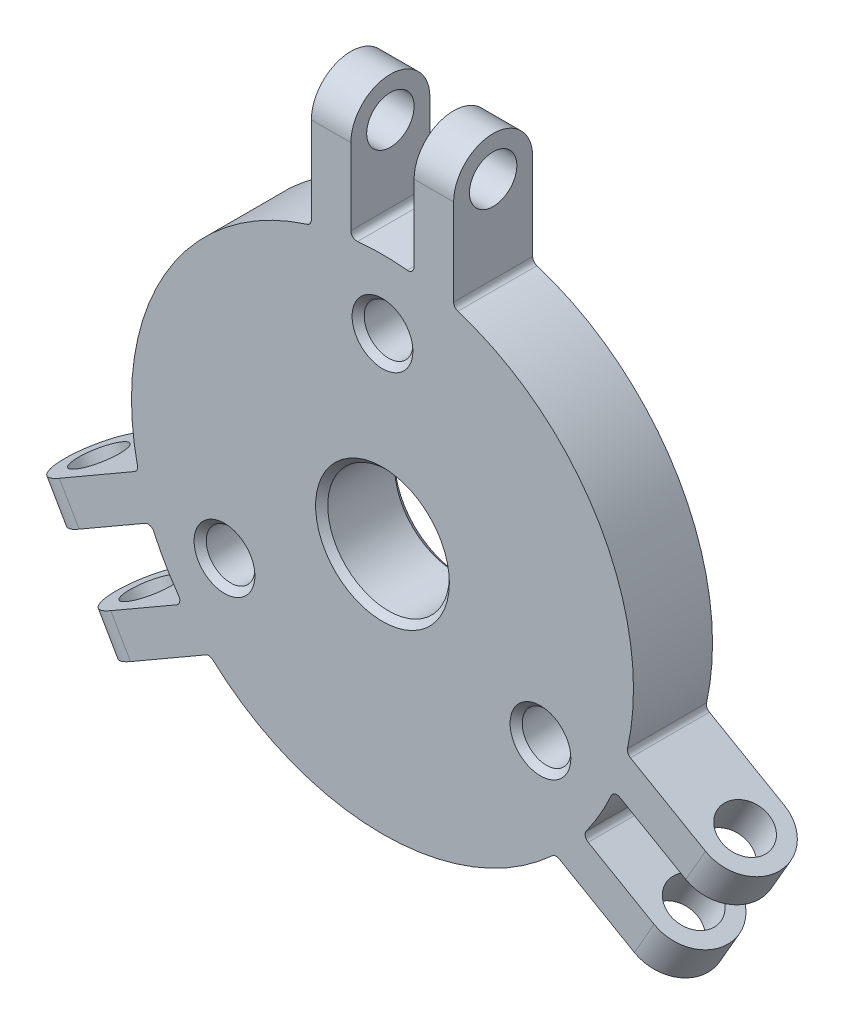
from build123d import *

# Parameters (mm, degrees)
BOSS_EXTRUDE1_DEPTH = 5
SKETCH2_R           = 1.5
CUT_EXTRUDE1_DEPTH  = 15.5
CUT_EXTRUDE3_DEPTH  = 27
CIRPATTERN1_COUNT   = 3
CIRPATTERN2_COUNT   = 3
SCALE_RATIO_1_SCALE = 1.3
SKETCH5_R           = 5
CUT_EXTRUDE4_DEPTH  = 10
CHAMFER1_SIZE       = 0.5
SKETCH8_R           = 2
CUT_EXTRUDE5_DEPTH  = 10
CHAMFER2_SIZE       = 0.5
FILLET1_R           = 0.5


with BuildPart() as part:
    # Sketch1 → Boss-Extrude1 (new body)
    with BuildSketch(Plane.XY):
        with BuildLine():
            Line((-26.5, -17.60918321), (-12.640472866, -9.607381488))
            ThreePointArc((-12.640472866, -9.607381488), (-13.75, -7.938566201), (-14.640472866, -6.143279873))
            Line((-14.640472866, -6.143279873), (-28.5, -14.145081595))
            Line((-28.5, -14.145081595), (-29.75, -11.980018086))
            Line((-29.75, -11.980018086), (-15.436166994, -3.715922747))
            ThreePointArc((-15.436166994, -3.715922747), (-13.75, 7.938566201), (-4.5, 15.226074127))
            Line((-4.5, 15.226074127), (-4.5, 31.754264805))
            Line((-4.5, 31.754264805), (-2, 31.754264805))
            Line((-2, 31.754264805), (-2, 15.750661362))
            ThreePointArc((-2, 15.750661362), (0, 15.877132403), (2, 15.750661362))
            Line((2, 15.750661362), (2, 31.754264805))
            Line((2, 31.754264805), (4.5, 31.754264805))
            Line((4.5, 31.754264805), (4.5, 15.226074127))
            ThreePointArc((4.5, 15.226074127), (13.75, 7.938566201), (15.436166994, -3.715922747))
            Line((15.436166994, -3.715922747), (29.75, -11.980018086))
            Line((29.75, -11.980018086), (28.5, -14.145081595))
            Line((28.5, -14.145081595), (14.640472866, -6.143279873))
            ThreePointArc((14.640472866, -6.143279873), (13.75, -7.938566201), (12.640472866, -9.607381488))
            Line((12.640472866, -9.607381488), (26.5, -17.60918321))
            Line((26.5, -17.60918321), (25.25, -19.77424672))
            Line((25.25, -19.77424672), (10.936166994, -11.510151381))
            ThreePointArc((10.936166994, -11.510151381), (0, -15.877132403), (-10.936166994, -11.510151381))
            Line((-10.936166994, -11.510151381), (-25.25, -19.77424672))
            Line((-25.25, -19.77424672), (-26.5, -17.60918321))
        make_face()
    extrude(amount=BOSS_EXTRUDE1_DEPTH)

    # Sketch2 → Cut-Extrude1 (cut, symmetric)
    with BuildSketch(Plane(origin=(0, 0, 0), x_dir=(0, 0, -1), z_dir=(1, 0, 0))):
        with Locations(Location((-2.5, 21, 0), (0, 0, 90))):
            Circle(SKETCH2_R)
    cut_extrude1 = extrude(amount=CUT_EXTRUDE1_DEPTH, both=True, mode=Mode.SUBTRACT)

    # Sketch4 → Cut-Extrude3 (cut)
    with BuildSketch(Plane.ZY.offset(4.5)):
        with BuildLine():
            Line((0, 21), (0, 31.754264805))
            Line((0, 31.754264805), (5, 31.754264805))
            Line((5, 31.754264805), (5, 21))
            ThreePointArc((5, 21), (2.5, 23.5), (0, 21))
        make_face()
    cut_extrude3 = extrude(amount=-CUT_EXTRUDE3_DEPTH, mode=Mode.SUBTRACT)

    # CirPattern1: Cut-Extrude3 ×3 about axis
    cirpattern1_axis = Axis((0, 0, 5), (0, 0, -1))
    for i in range(1, CIRPATTERN1_COUNT):
        add(cut_extrude3.rotate(cirpattern1_axis, i * 360 / CIRPATTERN1_COUNT), mode=Mode.SUBTRACT)

    # CirPattern2: Cut-Extrude1 ×3 about axis
    cirpattern2_axis = Axis((0, 0, 5), (0, 0, -1))
    for i in range(1, CIRPATTERN2_COUNT):
        add(cut_extrude1.rotate(cirpattern2_axis, i * 360 / CIRPATTERN2_COUNT), mode=Mode.SUBTRACT)


with BuildPart() as part_1:
    # Scale ratio 1: scaled about (0, 0, 2.5)
    add(part.part.scale(SCALE_RATIO_1_SCALE).moved(Location((0, 0, -0.75))))

    # Sketch5 → Cut-Extrude4 (cut)
    with BuildSketch(Plane.XY.offset(5.75)):
        Circle(SKETCH5_R)
    extrude(amount=-CUT_EXTRUDE4_DEPTH, mode=Mode.SUBTRACT)

    # Chamfer1
    chamfer1_edges = [part_1.edges().sort_by_distance(p)[0] for p in [
        (-5, 0, -0.75),
        (-5, 0, 5.75),
    ]]
    chamfer(chamfer1_edges, length=CHAMFER1_SIZE)

    # Sketch8 → Cut-Extrude5 (cut)
    with BuildSketch(Plane.XY.offset(5.75)):
        with Locations((0, 15)):
            Circle(SKETCH8_R)
        with Locations((12.990381057, -7.5)):
            Circle(SKETCH8_R)
        with Locations((-12.990381057, -7.5)):
            Circle(SKETCH8_R)
    extrude(amount=-CUT_EXTRUDE5_DEPTH, mode=Mode.SUBTRACT)

    # Chamfer2
    chamfer2_edges = [part_1.edges().sort_by_distance(p)[0] for p in [
        (-2, 15, -0.75),
        (-2, 15, 5.75),
        (10.990381057, -7.5, -0.75),
        (10.990381057, -7.5, 5.75),
        (-14.990381057, -7.5, -0.75),
        (-14.990381057, -7.5, 5.75),
    ]]
    chamfer(chamfer2_edges, length=CHAMFER2_SIZE)

    # Fillet1
    fillet1_edges = [part_1.edges().sort_by_distance(p)[0] for p in [
        (-16.432614725, -12.489595935, 2.5),
        (-19.032614725, -7.986263835, 2.5),
        (-20.067017093, -4.830699571, 2.5),
        (-5.85, 19.793896366, 2.5),
        (-2.6, 20.47585977, 2.5),
        (2.6, 20.47585977, 2.5),
        (5.85, 19.793896366, 2.5),
        (20.067017093, -4.830699571, 2.5),
        (19.032614725, -7.986263835, 2.5),
        (16.432614725, -12.489595935, 2.5),
        (14.217017093, -14.963196795, 2.5),
        (-14.217017093, -14.963196795, 2.5),
    ]]
    fillet(fillet1_edges, radius=FILLET1_R)


solid = part_1.part
